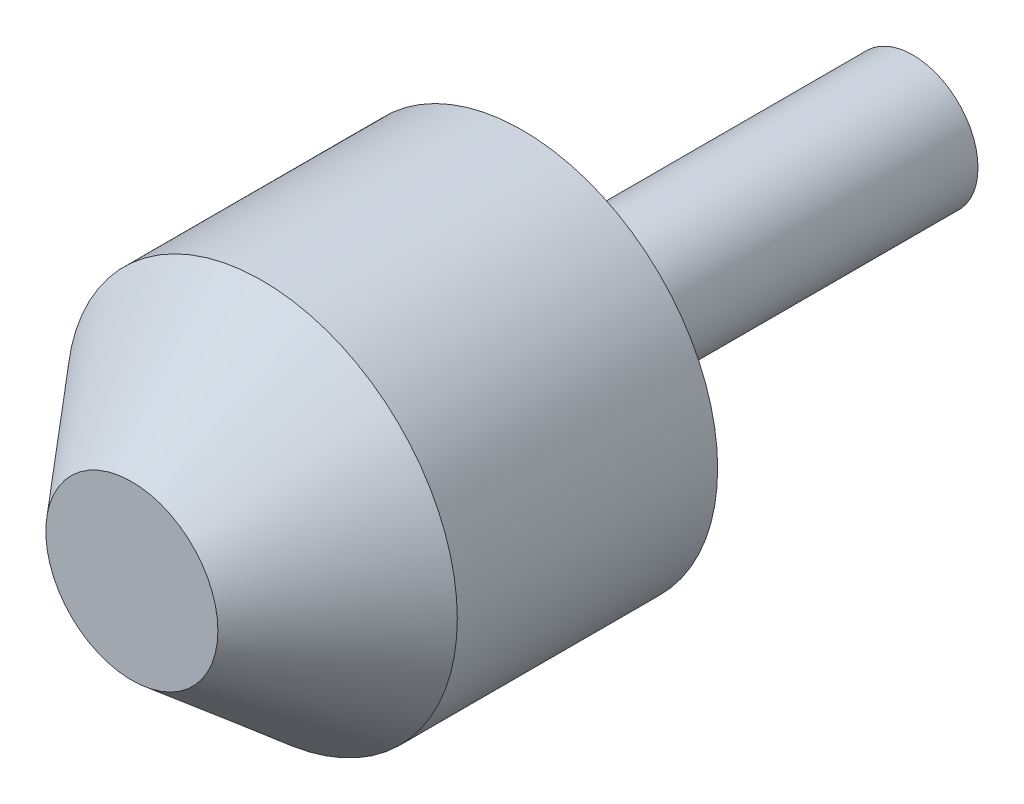
SolidWorks part; units mm, degrees
material "PVC Rigid"
ref_plane "Front Plane" through (0, 0, 0) normal (0, 0, 1) x (1, 0, 0)
ref_plane "Top Plane" through (0, 0, 0) normal (0, 1, 0) x (1, 0, 0)
ref_plane "Right Plane" through (0, 0, 0) normal (1, 0, 0) x (0, 0, -1)
sketch "Sketch1" plane through (0, 0, 0) normal (0, 0, 1) x (1, 0, 0)
  circle A0 centre (0, 0) radius 5
  dimension "D1" = 10
extrude "Boss-Extrude1" add sketch "Sketch1" along normal blind 30
sketch "Sketch2" plane through (0, 0, 30) normal (0, 0, 1) x (1, 0, 0)
  circle A0 centre (0, 0) radius 15
  dimension "D1" = 30
extrude "Boss-Extrude2" add sketch "Sketch2" along normal blind 30
chamfer "Chamfer1" distance 10 angle 40 1 edges at (15, 0, 60)
